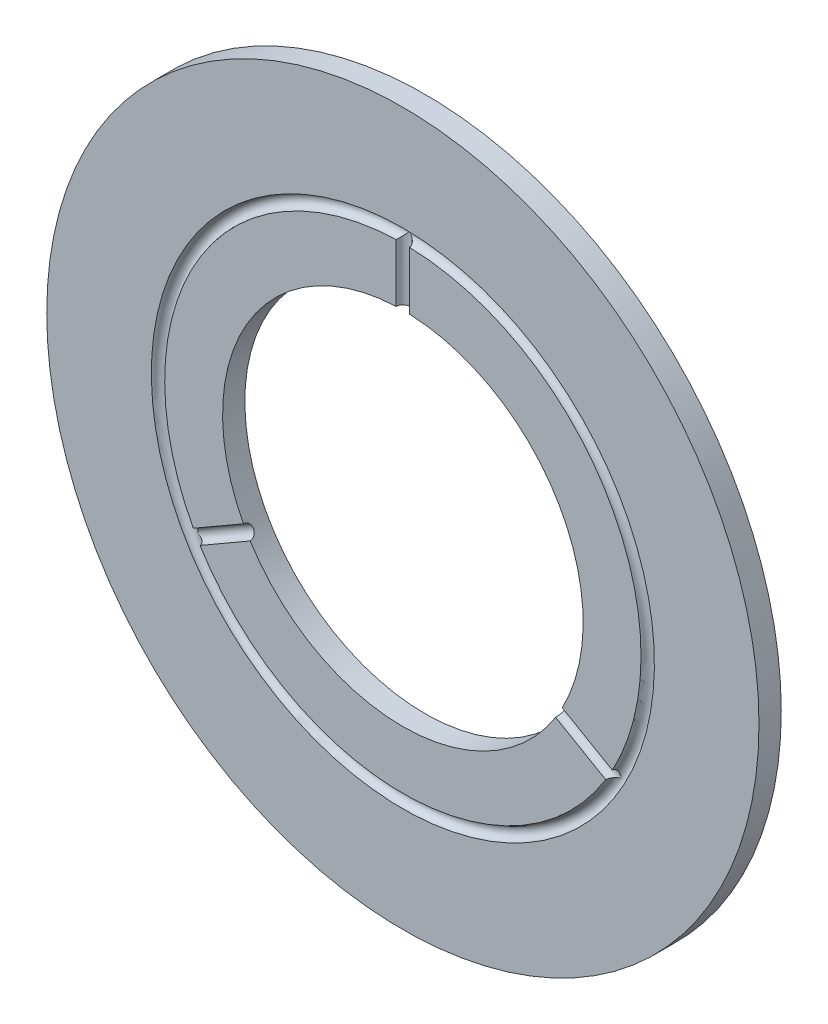
from build123d import *

# Parameters (mm, degrees)
SKETCH_1_R               = 80
SKETCH_1_R_2             = 40.5
EXTRUDE_1_DEPTH          = 5
SKETCH_3_R               = 1.5
SKETCH_5_R               = 1.5
CUT_EXTRUDE_2_DEPTH      = 55
PATTERN_CIRCULAR_1_COUNT = 3


with BuildPart() as part:
    # 草图1 → 凸台-拉伸1 (new body)
    with BuildSketch(Plane.XY):
        Circle(SKETCH_1_R)
        Circle(SKETCH_1_R_2, mode=Mode.SUBTRACT)
    extrude(amount=EXTRUDE_1_DEPTH)

    # 切除-扫描1: sweep along a path in 草图2
    with BuildLine(Plane.XY.offset(5)) as sweep_1_path:
        CenterArc((0, 0), 55, 0, 360)
    # 草图3 → 切除-扫描1 (sweep, cut)
    with BuildSketch(Plane(origin=(0, 0, 0), x_dir=(0, 0, -1), z_dir=(1, 0, 0))):
        with Locations((-5, 55)):
            Circle(SKETCH_3_R)
    sweep(path=sweep_1_path.line, mode=Mode.SUBTRACT)

    # 草图5 → 切除-拉伸2 (cut)
    with BuildSketch(Plane(origin=(0, 0, 0), x_dir=(1, 0, 0), z_dir=(0, 1, 0))):
        with Locations((0, -5)):
            Circle(SKETCH_5_R)
    cut_extrude_2 = extrude(amount=CUT_EXTRUDE_2_DEPTH, mode=Mode.SUBTRACT)

    # 阵列(圆周)1: 切除-拉伸2 ×3 about axis
    pattern_circular_1_axis = Axis((0, 0, 5), (0, 0, -1))
    for i in range(1, PATTERN_CIRCULAR_1_COUNT):
        add(cut_extrude_2.rotate(pattern_circular_1_axis, i * 360 / PATTERN_CIRCULAR_1_COUNT), mode=Mode.SUBTRACT)


solid = part.part
